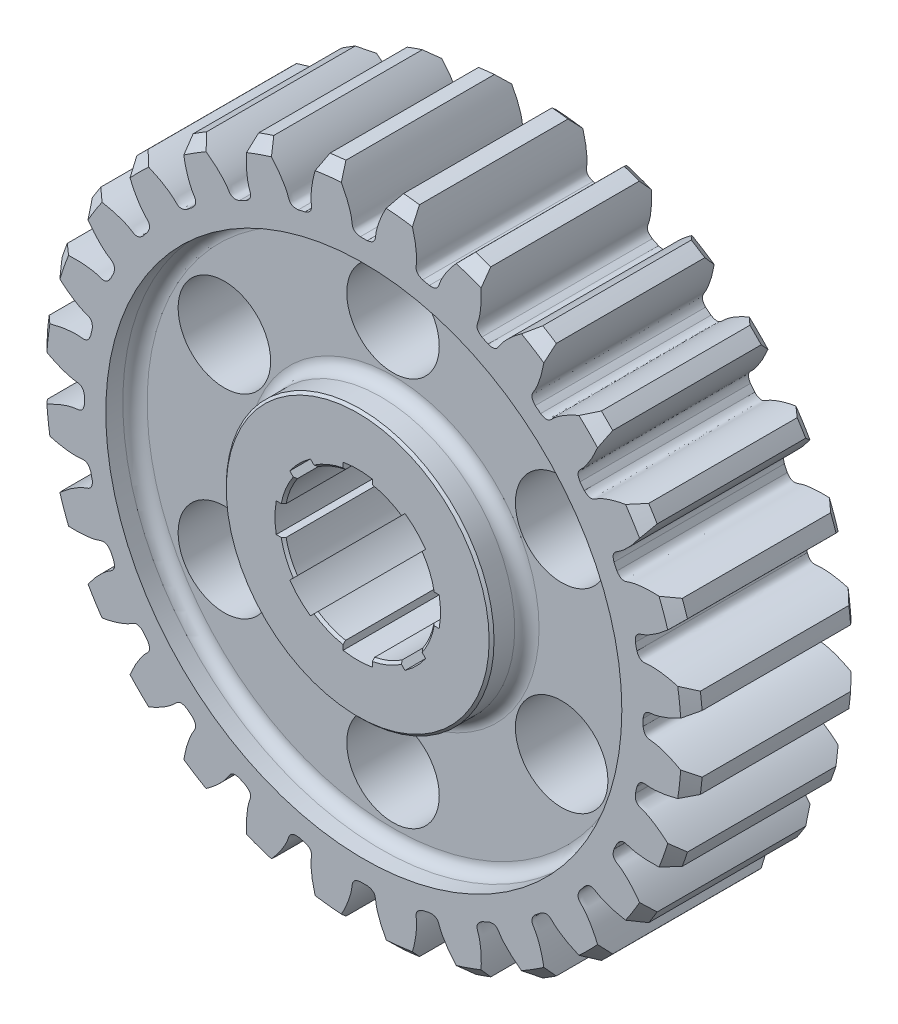
from build123d import *

# Parameters (mm, degrees)
SKETCH_1_R               = 135
EXTRUDE_1_DEPTH          = 70
CHAMFER_1_SIZE           = 4.5
CUT_EXTRUDE_1_DEPTH      = 204.346994077
PATTERN_CIRCULAR_1_COUNT = 28
EXTRUDE_2_DEPTH          = 72.5
EXTRUDE_2_DEPTH_BACK     = 2.5
SKETCH_4_R               = 55
CHAMFER_2_SIZE           = 1
CHAMFER_3_SIZE           = 1
SKETCH_5_R               = 19
CUT_EXTRUDE_2_DEPTH      = 204.532776826
PATTERN_CIRCULAR_2_COUNT = 6
SKETCH_7_R               = 31
CUT_EXTRUDE_3_DEPTH      = 205.436643591
CHAMFER_4_SIZE           = 1
CHAMFER_5_SIZE           = 1
CUT_EXTRUDE_4_DEPTH      = 170


with BuildPart() as part:
    # 草图1 → 凸台-拉伸1 (new body)
    with BuildSketch(Plane.XY):
        Circle(SKETCH_1_R)
    extrude(amount=EXTRUDE_1_DEPTH)

    # 倒角1
    chamfer_1_edges = [part.edges().sort_by_distance(p)[0] for p in [
        (-135, 0, 0),
        (-135, 0, 70),
    ]]
    chamfer(chamfer_1_edges, length=CHAMFER_1_SIZE)

    # 草图2 → 切除-拉伸1 (cut, through all)
    with BuildSketch(Plane.XY):
        with BuildLine():
            ThreePointArc((1.409502014, 114.741343046), (0, 114.75), (-1.409502014, 114.741343046))
            add(Edge.make_bspline(
                [(-1.409502014, 114.741343046), (-4.898074499, 115.196836625), (-4.677516338, 117.168119441), (-4.984398895, 119.162291727), (-5.037036609, 119.465620008), (-5.104798185, 119.814317811), (-5.189428257, 120.207906411), (-5.292774003, 120.645824391), (-5.416628774, 121.127464638), (-5.56278081, 121.652162891), (-5.732995865, 122.219201961), (-5.929020731, 122.827811049), (-6.152580285, 123.47716663), (-6.405376537, 124.166392908), (-6.689087098, 124.894562441), (-7.005363833, 125.660696769), (-7.355831483, 126.463767078), (-7.742086319, 127.302694902), (-8.165694807, 128.176352857), (-8.628192292, 129.08356541), (-9.131081705, 130.023109676), (-9.675832282, 130.993716255), (-10.263878312, 131.994070096), (-10.896617901, 133.022811393), (-11.575411759, 134.078536512), (-12.30158201, 135.159798952), (-13.076411029, 136.26511033), (-13.901140295, 137.392941404), (-14.776969276, 138.54172311), (-15.705054338, 139.709847649), (-16.686507681, 140.895669577), (-17.722396296, 142.097506946), (-18.813740962, 143.313642451), (-19.961515254, 144.542324614), (-21.166644603, 145.781768995), (-22.430005339, 147.030159416), (-23.752423916, 148.285649218), (-25.134675597, 149.546362555), (-27.082171902, 151.25254709), (-28.599475372, 152.502513665), (-29.639240308, 153.325554502)],
                knots=[0, 0, 0, 0, 0.112672291, 0.1180235, 0.124347656, 0.131644759, 0.139914809, 0.149157806, 0.15937375, 0.170562641, 0.182724479, 0.195859265, 0.209966997, 0.225047676, 0.241101302, 0.258127876, 0.276127396, 0.295099864, 0.315045278, 0.33596364, 0.357854948, 0.380719204, 0.404556407, 0.429366557, 0.455149653, 0.481905697, 0.509634688, 0.538336626, 0.568011511, 0.598659343, 0.630280122, 0.662873848, 0.696440521, 0.730980141, 0.766492709, 0.802978223, 0.840436684, 0.878868093, 0.918272448, 1, 1, 1, 1], degree=3))
            ThreePointArc((-29.639240308, 153.325554502), (0, 156.164049094), (29.639240308, 153.325554502))
            add(Edge.make_bspline(
                [(1.409502014, 114.741343046), (4.898074499, 115.196836625), (4.677516338, 117.168119441), (4.984398895, 119.162291727), (5.037036609, 119.465620008), (5.104798185, 119.814317811), (5.189428257, 120.207906411), (5.292774003, 120.645824391), (5.416628774, 121.127464638), (5.56278081, 121.652162891), (5.732995865, 122.219201961), (5.929020731, 122.827811049), (6.152580285, 123.47716663), (6.405376537, 124.166392908), (6.689087098, 124.894562441), (7.005363833, 125.660696769), (7.355831483, 126.463767078), (7.742086319, 127.302694902), (8.165694807, 128.176352857), (8.628192292, 129.08356541), (9.131081705, 130.023109676), (9.675832282, 130.993716255), (10.263878312, 131.994070096), (10.896617901, 133.022811393), (11.575411759, 134.078536512), (12.30158201, 135.159798952), (13.076411029, 136.26511033), (13.901140295, 137.392941404), (14.776969276, 138.54172311), (15.705054338, 139.709847649), (16.686507681, 140.895669577), (17.722396296, 142.097506946), (18.813740962, 143.313642451), (19.961515254, 144.542324614), (21.166644603, 145.781768995), (22.430005339, 147.030159416), (23.752423916, 148.285649218), (25.134675597, 149.546362555), (27.082171902, 151.25254709), (28.599475372, 152.502513665), (29.639240308, 153.325554502)],
                knots=[0, 0, 0, 0, 0.112672291, 0.1180235, 0.124347656, 0.131644759, 0.139914809, 0.149157806, 0.15937375, 0.170562641, 0.182724479, 0.195859265, 0.209966997, 0.225047676, 0.241101302, 0.258127876, 0.276127396, 0.295099864, 0.315045278, 0.33596364, 0.357854948, 0.380719204, 0.404556407, 0.429366557, 0.455149653, 0.481905697, 0.509634688, 0.538336626, 0.568011511, 0.598659343, 0.630280122, 0.662873848, 0.696440521, 0.730980141, 0.766492709, 0.802978223, 0.840436684, 0.878868093, 0.918272448, 1, 1, 1, 1], degree=3))
        make_face()
    cut_extrude_1 = extrude(amount=CUT_EXTRUDE_1_DEPTH, mode=Mode.SUBTRACT)

    # 阵列(圆周)1: 切除-拉伸1 ×28 about axis
    pattern_circular_1_axis = Axis((0, 0, 70), (0, 0, -1))
    for i in range(1, PATTERN_CIRCULAR_1_COUNT):
        add(cut_extrude_1.rotate(pattern_circular_1_axis, i * 360 / PATTERN_CIRCULAR_1_COUNT), mode=Mode.SUBTRACT)

    # 草图4 → 凸台-拉伸2 (add, two sides: drawn at the far end of the back side and taken through both)
    with BuildSketch(Plane.XY.offset(-EXTRUDE_2_DEPTH_BACK)):
        Circle(SKETCH_4_R)
    extrude(amount=EXTRUDE_2_DEPTH + EXTRUDE_2_DEPTH_BACK)

    # 倒角2
    chamfer_2_edges = [part.edges().sort_by_distance(p)[0] for p in [
        (-55, 0, 72.5),
    ]]
    chamfer(chamfer_2_edges, length=CHAMFER_2_SIZE)

    # 倒角3
    chamfer_3_edges = [part.edges().sort_by_distance(p)[0] for p in [
        (-55, 0, -2.5),
    ]]
    chamfer(chamfer_3_edges, length=CHAMFER_3_SIZE)

    # 草图5 → 切除-拉伸2 (cut, through all)
    with BuildSketch(Plane.XY):
        with Locations((0, 80)):
            Circle(SKETCH_5_R)
    cut_extrude_2 = extrude(amount=CUT_EXTRUDE_2_DEPTH, mode=Mode.SUBTRACT)

    # 阵列(圆周)2: 切除-拉伸2 ×6 about axis
    pattern_circular_2_axis = Axis((0, 0, 0), (0, 0, 1))
    for i in range(1, PATTERN_CIRCULAR_2_COUNT):
        add(cut_extrude_2.rotate(pattern_circular_2_axis, i * 360 / PATTERN_CIRCULAR_2_COUNT), mode=Mode.SUBTRACT)

    # 草图6 → 切除-旋转1 (revolve, cut)
    with BuildSketch(Plane(origin=(0, 0, 0), x_dir=(0, 0, -1), z_dir=(1, 0, 0)), mode=Mode.PRIVATE) as cut_revolve_1_sk:
        with BuildLine():
            Line((0, 106), (-7, 106))
            ThreePointArc((-7, 106), (-10.535533906, 104.535533906), (-12, 101))
            Line((-12, 101), (-12, 60))
            ThreePointArc((-12, 60), (-10.535533906, 56.464466094), (-7, 55))
            Line((-7, 55), (0, 55))
            Line((0, 55), (0, 106))
        make_face()
    cut_revolve_1 = revolve(cut_revolve_1_sk.sketch.rotate(Axis((0, 0, -0.679141344), (0, 0, -1)), 90), axis=Axis((0, 0, -0.679141344), (0, 0, -1)), mode=Mode.SUBTRACT)

    # 草图7 → 切除-拉伸3 (cut, through all)
    with BuildSketch(Plane.XY.offset(-2.5)):
        Circle(SKETCH_7_R)
    extrude(amount=CUT_EXTRUDE_3_DEPTH, mode=Mode.SUBTRACT)

    # 倒角4
    chamfer_4_edges = [part.edges().sort_by_distance(p)[0] for p in [
        (-31, 0, -2.5),
    ]]
    chamfer(chamfer_4_edges, length=CHAMFER_4_SIZE)

    # 倒角5
    chamfer_5_edges = [part.edges().sort_by_distance(p)[0] for p in [
        (-31, 0, 72.5),
    ]]
    chamfer(chamfer_5_edges, length=CHAMFER_5_SIZE)

    # 镜向1: 切除-旋转1 across plane
    add(cut_revolve_1.mirror(Plane(origin=(0, 0, 35), x_dir=(1, 0, 0), z_dir=(0, 0, -1))), mode=Mode.SUBTRACT)

    # 草图10 → 切除-拉伸4 (cut)
    with BuildSketch(Plane(origin=(0, 0, -2.5), x_dir=(-1, 0, 0), z_dir=(0, 0, -1))):
        with BuildLine():
            Line((-6, 33.466401061), (-6, 30.413812651))
            ThreePointArc((-6, 30.413812651), (-11.863186403, 28.640265508), (-17.26317248, 25.748453855))
            Line((-17.26317248, 25.748453855), (-19.421678445, 27.90695982))
            ThreePointArc((-19.421678445, 27.90695982), (-24.04163056, 24.04163056), (-27.90695982, 19.421678445))
            Line((-27.90695982, 19.421678445), (-25.748453855, 17.26317248))
            ThreePointArc((-25.748453855, 17.26317248), (-28.640265508, 11.863186403), (-30.413812651, 6))
            Line((-30.413812651, 6), (-33.466401061, 6))
            ThreePointArc((-33.466401061, 6), (-34, 0), (-33.466401061, -6))
            Line((-33.466401061, -6), (-30.413812651, -6))
            ThreePointArc((-30.413812651, -6), (-28.640265508, -11.863186403), (-25.748453855, -17.26317248))
            Line((-25.748453855, -17.26317248), (-27.90695982, -19.421678445))
            ThreePointArc((-27.90695982, -19.421678445), (-24.04163056, -24.04163056), (-19.421678445, -27.90695982))
            Line((-19.421678445, -27.90695982), (-17.26317248, -25.748453855))
            ThreePointArc((-17.26317248, -25.748453855), (-11.863186403, -28.640265508), (-6, -30.413812651))
            Line((-6, -30.413812651), (-6, -33.466401061))
            ThreePointArc((-6, -33.466401061), (0, -34), (6, -33.466401061))
            Line((6, -33.466401061), (6, -30.413812651))
            ThreePointArc((6, -30.413812651), (11.863186403, -28.640265508), (17.26317248, -25.748453855))
            Line((17.26317248, -25.748453855), (19.421678445, -27.90695982))
            ThreePointArc((19.421678445, -27.90695982), (24.04163056, -24.04163056), (27.90695982, -19.421678445))
            Line((27.90695982, -19.421678445), (25.748453855, -17.26317248))
            ThreePointArc((25.748453855, -17.26317248), (28.640265508, -11.863186403), (30.413812651, -6))
            Line((30.413812651, -6), (33.466401061, -6))
            ThreePointArc((33.466401061, -6), (34, 0), (33.466401061, 6))
            Line((33.466401061, 6), (30.413812651, 6))
            ThreePointArc((30.413812651, 6), (28.640265508, 11.863186403), (25.748453855, 17.26317248))
            Line((25.748453855, 17.26317248), (27.90695982, 19.421678445))
            ThreePointArc((27.90695982, 19.421678445), (24.04163056, 24.04163056), (19.421678445, 27.90695982))
            Line((19.421678445, 27.90695982), (17.26317248, 25.748453855))
            ThreePointArc((17.26317248, 25.748453855), (11.863186403, 28.640265508), (6, 30.413812651))
            Line((6, 30.413812651), (6, 33.466401061))
            ThreePointArc((6, 33.466401061), (0, 34), (-6, 33.466401061))
        make_face()
    extrude(amount=-CUT_EXTRUDE_4_DEPTH, mode=Mode.SUBTRACT)


solid = part.part
